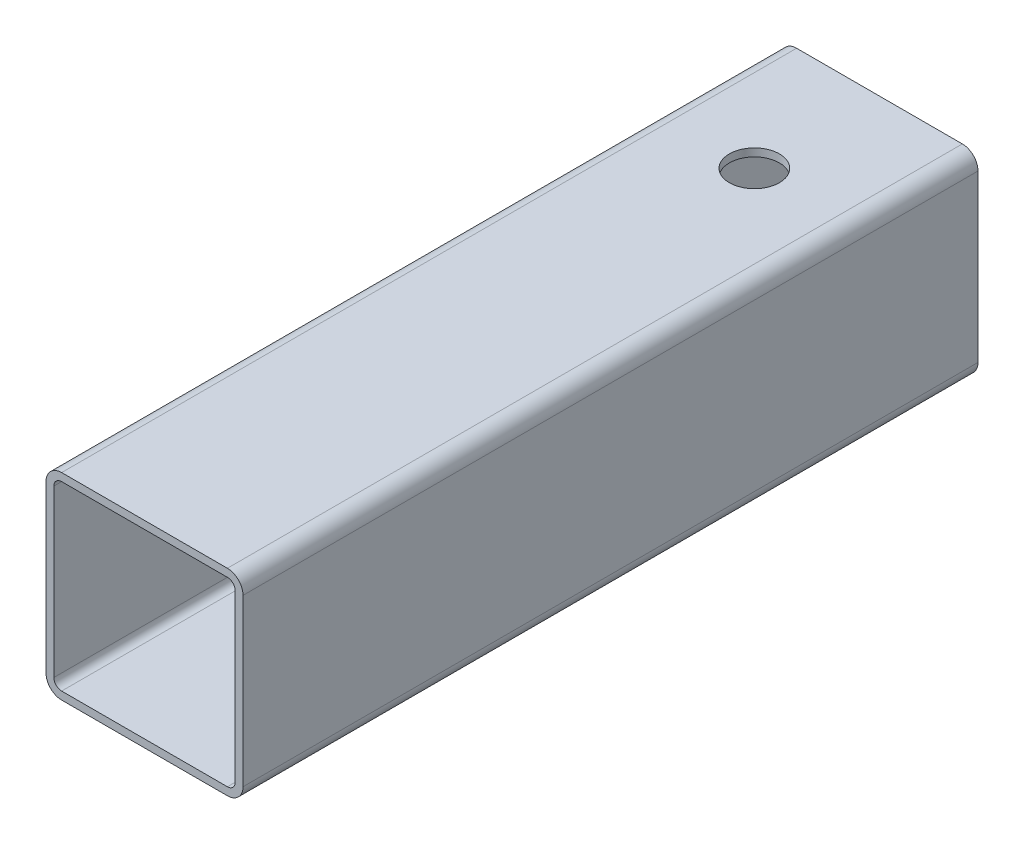
from build123d import *

# Parameters (mm, degrees)
BOSS_EXTRUDE1_DEPTH     = 235
CUT_EXTRUDE1_DEPTH      = 252.322501977
CUT_EXTRUDE1_DEPTH_BACK = 252.322501977
SKETCH_1_R              = 16


with BuildPart() as part:
    # Sketch1 → Boss-Extrude1 (new, symmetric)
    with BuildSketch(Plane.XY):
        with BuildLine():
            Line((-53, -63), (53, -63))
            ThreePointArc((53, -63), (60.071067812, -60.071067812), (63, -53))
            Line((63, -53), (63, 53))
            ThreePointArc((63, 53), (60.071067812, 60.071067812), (53, 63))
            Line((53, 63), (-53, 63))
            ThreePointArc((-53, 63), (-60.071067812, 60.071067812), (-63, 53))
            Line((-63, 53), (-63, -53))
            ThreePointArc((-63, -53), (-60.071067812, -60.071067812), (-53, -63))
        make_face()
        with BuildLine():
            Line((-53, -58), (53, -58))
            ThreePointArc((53, -58), (56.535533906, -56.535533906), (58, -53))
            Line((58, -53), (58, 53))
            ThreePointArc((58, 53), (56.535533906, 56.535533906), (53, 58))
            Line((53, 58), (-53, 58))
            ThreePointArc((-53, 58), (-56.535533906, 56.535533906), (-58, 53))
            Line((-58, 53), (-58, -53))
            ThreePointArc((-58, -53), (-56.535533906, -56.535533906), (-53, -58))
        make_face(mode=Mode.SUBTRACT)
    extrude(amount=BOSS_EXTRUDE1_DEPTH, both=True)

    # 草图1 → Cut-Extrude1 (cut, two sides: drawn at the far end of the back side and taken through both)
    with BuildSketch(Plane(origin=(0, 0, 0), x_dir=(1, 0, 0), z_dir=(0, 1, 0)).offset(-CUT_EXTRUDE1_DEPTH_BACK)):
        with Locations(Location((0, 155, 0), (0, 0, 270))):
            Circle(SKETCH_1_R)
    extrude(amount=CUT_EXTRUDE1_DEPTH + CUT_EXTRUDE1_DEPTH_BACK, mode=Mode.SUBTRACT)


solid = part.part
